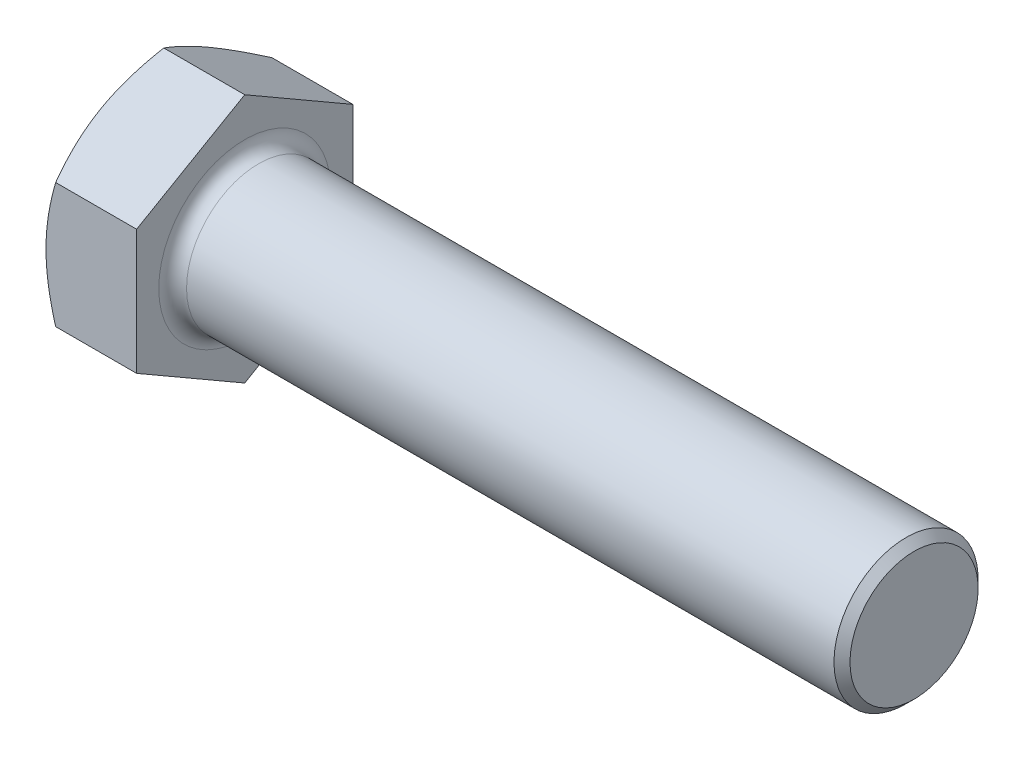
SolidWorks part; units mm, degrees
material "Q235"
ref_plane "Front Plane" through (0, 0, 0) normal (0, 0, 1) x (1, 0, 0)
ref_plane "Top Plane" through (0, 0, 0) normal (0, 1, 0) x (1, 0, 0)
ref_plane "Right Plane" through (0, 0, 0) normal (1, 0, 0) x (0, 0, -1)
sketch "Sketch1" plane through (0, 0, 0) normal (0, 0, 1) x (1, 0, 0)
  line L0 (0, 0) -> (73.8, 0) construction
  line L1 (0, 0) -> (0, 11.39)
  line L2 (0, 11.39) -> (8.8, 11.39)
  line L3 (8.8, 11.39) -> (8.8, 0)
  line L4 (8.8, 7) -> (73.8, 7)
  line L5 (73.8, 7) -> (73.8, 0)
  line L6 (0, 10.5) -> (0.5138, 11.39)
  line L7 (69.8, 7) -> (69.8, 0)
  line L8 (14.8, 7) -> (14.8, 0)
  line L9 (8.8, 6.3505) -> (73.8, 6.3505)
  line L10 (73.8, 5.9175) -> (8.8, 5.9175)
  line L11 (8.2, 10.075) -> (8.8, 9.475)
  line L12 (8.2, 11.39) -> (8.2, 0)
  line L13 (8.7, 9.575) -> (8.7, 0) construction
  arc A0 (8.8, 8.35) -> (10.15, 7) centre (10.15, 8.35) ccw
  point P12 (71.8, 0)
  point P13 (2.95, 11.39)
  point P14 (8.8, 8.35)
  point P24 (8.8, 9.575)
  dimension "D1" = 0.1
  dimension "r" = 1.35
  dimension "k" = 8.8
  dimension "D2" = 45
  dimension "β" = 30
  dimension "e" = 22.78
  dimension "s" = 21
  dimension "d" = 14
  dimension "l" = 65
  dimension "D52" = 4
  dimension "P" = 2
  dimension "kw" = 5.85
  dimension "da" = 16.7
  dimension "a" = 6
  dimension "ds" = 12.701
  dimension "D61" = 11.835
  dimension "dw" = 19.15
  dimension "c" = 0.6
sketch "Sketch2" plane through (0, 0, 0) normal (1, 0, 0) x (0, 0, -1)
  line L1 (0, 12.1244) -> (-10.5, 6.0622)
  line L2 (-10.5, 6.0622) -> (-10.5, -6.0622)
  line L3 (-10.5, -6.0622) -> (0, -12.1244)
  line L4 (0, -12.1244) -> (10.5, -6.0622)
  line L5 (10.5, -6.0622) -> (10.5, 6.0622)
  line L6 (10.5, 6.0622) -> (0, 12.1244)
  circle A0 centre (0, 0) radius 10.5 construction
sketch "Sketch3" plane through (0, 0, 0) normal (1, 0, 0) x (0, 0, -1)
  line L0 (10.5, 6.0622) -> (0, 12.1244) construction
  line L1 (0, 12.1244) -> (-10.5, 6.0622) construction
  line L2 (-10.5, 6.0622) -> (-10.5, -6.0622) construction
  line L3 (10.5, -6.0622) -> (10.5, 6.0622) construction
  line L4 (0, -12.1244) -> (10.5, -6.0622) construction
  line L5 (-10.5, -6.0622) -> (0, -12.1244) construction
  line L6 (10.5, 6.0622) -> (0, 12.1244)
  line L7 (0, 12.1244) -> (-10.5, 6.0622)
  line L8 (-10.5, 6.0622) -> (-10.5, -6.0622)
  line L9 (10.5, -6.0622) -> (10.5, 6.0622)
  line L10 (0, -12.1244) -> (10.5, -6.0622)
  line L11 (-10.5, -6.0622) -> (0, -12.1244)
extrude "Boss-Extrude1" add sketch "Sketch3" along normal up to vertex (8.8 mm away) up to point (8.8, 11.39, 0)
sketch "Sketch4" plane through (0, 0, 0) normal (-1, 0, 0) x (0, 0, 1)
  circle A0 centre (0, 0) radius 10.5 construction
  circle A1 centre (0, 0) radius 10.5
  circle A2 centre (0, 0) radius 22.78
  dimension "D1" = 45.56
extrude "Cut-Extrude1" cut sketch "Sketch4" against normal blind 1.1 draft 60
sketch "Sketch5" plane through (0, 0, 0) normal (0, 0, 1) x (1, 0, 0)
  line L0 (8.8, 7) -> (73.8, 7) construction
  line L1 (73.8, 7) -> (73.8, 0) construction
  line L2 (0, 0) -> (73.8, 0) construction
  line L3 (10.15, 7) -> (73.8, 7)
  line L4 (73.8, 7) -> (73.8, 0)
  line L5 (8.8, 0) -> (73.8, 0)
  line L6 (8.8, 8.35) -> (8.8, 0)
  arc A0 (8.8, 8.35) -> (10.15, 7) centre (10.15, 8.35) ccw construction
  arc A1 (8.8, 8.35) -> (10.15, 7) centre (10.15, 8.35) ccw
revolve "Revolve1" add sketch "Sketch5" angle 360 about L5
cosmetic thread "Cosmetic Thread2" parameters "D1"=34, "D2"=11.835
chamfer "Chamfer2" distance 0.7778 angle 45 1 edges at (73.8, 0, 7)
sketch "Sketch7" plane through (0, 0, 0) normal (0, 0, 1) x (1, 0, 0)
  line L0 (8.8, 9.475) -> (8.2, 10.075)
  line L1 (8.2, 10.075) -> (8.2, 22.78)
  line L2 (8.2, 22.78) -> (8.8, 22.78)
  line L3 (8.8, 22.78) -> (8.8, 9.475)
  line L4 (0, 0) -> (73.8, 0) construction
  line L5 (0, 0) -> (73.8, 0) construction
  dimension "D1" = 45.56
revolve "Cut-Revolve1" [suppressed] cut sketch "Sketch7" angle 360 mid plane about L5
sketch "Sketch6" [suppressed] plane through (0, 0, 0) normal (0, 0, 1) x (1, 0, 0)
  line L0 (5.9, 0) -> (5.9, 2.5) construction
  line L1 (5.9, 2.5) -> (13.5, 2.5)
  line L2 (13.5, 2.5) -> (13.5, 0)
  line L3 (5.9, 2.5) -> (4.069, 2.245)
  line L5 (3.5, 2.2402) -> (13.5, 2.2402) construction
  line L6 (3.5, 4.315) -> (3.5, 0) construction
  line L7 (3.5, 2.7402) -> (3.5, 0)
  line L8 (3.5, 0) -> (13.5, 0)
  arc A0 (4.069, 2.245) -> (3.5, 2.7402) centre (4, 2.7402) cw
  arc A1 (3.5, 3) -> (4, 2.5) centre (4, 3) ccw construction
revolve "Revolve2" add sketch "Sketch6" angle 360 about L8
cosmetic thread "Cosmetic Thread1" [suppressed] parameters "D1"=34, "D2"=11.835
chamfer "Chamfer1" [suppressed] distance 0.7778 angle 45
sketch "Sketch8" plane through (0, 0, 0) normal (0, 0, 1) x (1, 0, 0)
  line L0 (8.8, 9.475) -> (8.2, 10.075)
  line L1 (8.2, 10.075) -> (8.2, 22.78)
  line L2 (8.2, 22.78) -> (8.8, 22.78)
  line L3 (8.8, 22.78) -> (8.8, 9.475)
  line L4 (0, 0) -> (73.8, 0) construction
  line L5 (0, 0) -> (73.8, 0) construction
  dimension "D1" = 45.56
revolve "Cut-Revolve2" [suppressed] cut sketch "Sketch8" angle 360 mid plane about L5
